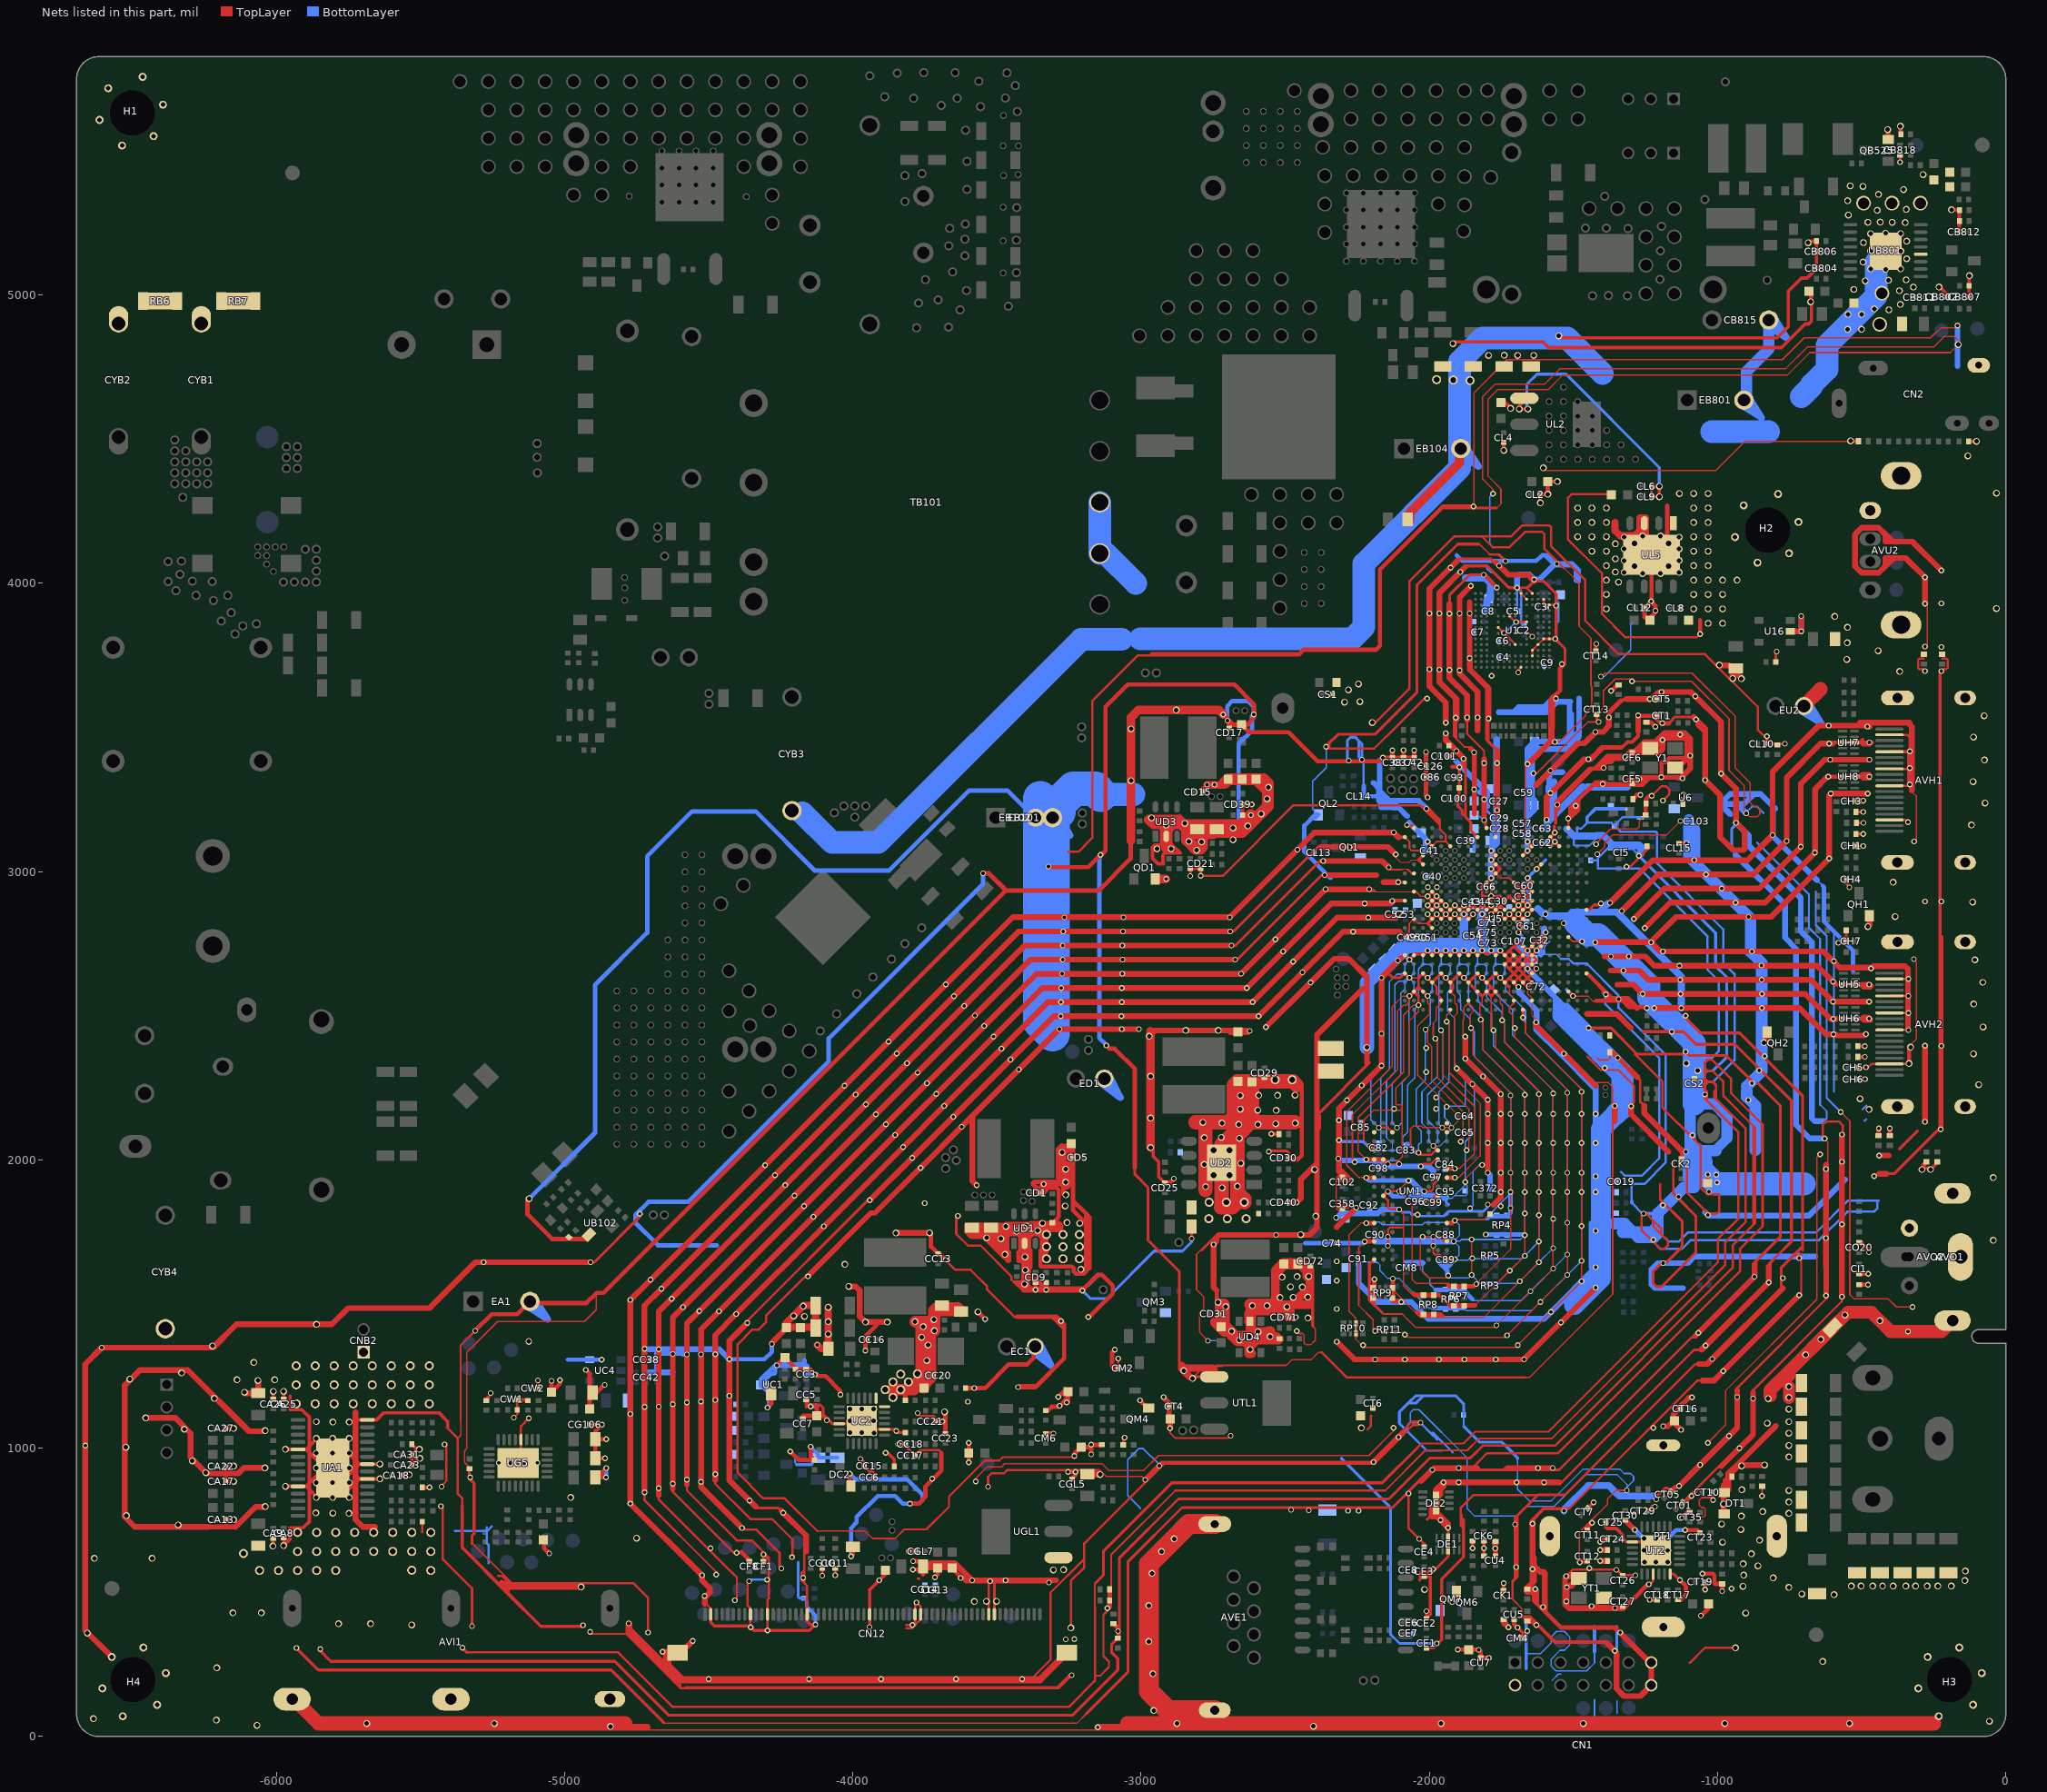
[diagram p0: the nets of this part, all layers, seen from the top]
# Altium PCB MISC84395.PcbDoc (part 18 of 26)
Units mil, origin at the board's own origin, x right, y up, seen from the top; angles counter-clockwise.
Board outline 6692.91 x 5826.77 mil, 2 copper layers (TopLayer, BottomLayer), stack 61.855 mil thick; 951 components, 565 nets, 4374 pads, 1804 vias.
Unrouted connection lines stored in the file: 1.

## Via types
v1: diameter 19.68, hole 11.81, TopLayer to BottomLayer, tented both sides, 1262 vias
v2: diameter 23.62, hole 15.75, TopLayer to BottomLayer, tented both sides, 524 vias
v3: diameter 31.5, hole 19.68, TopLayer to BottomLayer, tented both sides, 11 vias
v4: diameter 24, hole 16, TopLayer to BottomLayer, tented both sides, 6 vias
v5: diameter 19, hole 11.81, TopLayer to BottomLayer, tented both sides, 1 vias

## Nets (pads, with @x,y where several pads share a name; then routed paths per layer and width w, separated by ;. In a path a pad name is that pad's centre, name@x,y a point inside that pad or via, vN(x,y) a via of type N, cw(c..) or ccw(c..) an arc to the next point about the centre after c; other vN are vias at no path point) (continued)
GND: (continued)
  TopLayer w50: AVI1.2@-5931,123 -5853.5,45.5 v2(-5686,45.5) -5276,45.5 ; v2(-5243,45.5) -5276,45.5 ; -4790,45.5 -5276,45.5 ; -3048,45.5 v2(-2876,45.5) v2(-1959,45.5) v2(-1466,45.5) v2(-975,45.5) v2(-543,45.5) -249,45.5 ; -2811.57,2130.91 -2696.31,2130.91 -2678.73,2148.49 -2678.73,2259.08 -2665.51,2272.31 CD26.1@-2664.08,2272.31 ; v2@-2776.83,1896.05 -2776.83,2127.17 -2774,2130 -2679.22,2130 -2660.73,2148.49 -2660.73,2271.77 -2473.34,2271.77 -2460.57,2259 ; -2722.96,1835 -2721,1835 ; pad.VIA5@-2642,1853 -2642,1863.65 -2665.17,1886.83 ; CD28.1@-2615,2258 -2615,2159 -2721,2053 -2721,2033.31 UD2.9@-2721,1990 -2721,1946.69 -2721,1835 ; v2@-2466.98,2130.83 -2618.3,2130.83 -2665.17,2083.95 -2665.17,1886.83 ; EU2.2@-700.62,3574 -700.62,3575.38 -644,3632 ; -2721,1835 -2684,1835 -2665.17,1853.83 -2665.17,1886.83
  TopLayer w70: AVE1.9@-2744.49,91.34 -2906.34,91.34 -2973,158 v2(-2973,330) v2(-2973,454) -2973,598 v2(-2929,642) v2(-2885,686) -2833.99,737.01 AVE1.10@-2744.49,737.01
  BottomLayer w3.94: -2148.9,2077.23 -2128.24,2056.56 -2128.24,2031.45 ; -2120.36,2032.93 -2104.62,2032.93 ; -2085.42,2654.49 -2084.93,2654.98 -2084.93,2678.6 v1(-2069.18,2694.35) -2053.43,2678.6 -2053.43,2647.1 v1(-2069.18,2631.36) ; -2084.93,2591.99 -2084.93,2615.61 v1(-2069.18,2631.36) ; -2053.93,2583.62 -2053.43,2584.11 -2053.43,2615.61 v1(-2069.18,2631.36) ; v1(-2037.69,2536.87) -2037.69,2662.85 -2021.94,2678.6 ; -2021.94,2725.52 -2021.94,2710.1 -2021.94,2678.6 ; v1(-2006.19,2568.36) -1990.44,2584.11 -1990.44,2615.61 v1(-2006.19,2631.36) -1990.44,2647.1 -1990.44,2670.73 -1998.32,2678.6 -2021.94,2678.6 ; -2002.25,2072.3 -2002.25,2088.05 ; v1(-1986.51,2048.68) -1961.9,2048.68 -1939.26,2071.32 -1939.26,2088.37 -1923.51,2104.12 v1(-1923.51,2111.67) ; -1970.76,2072.3 -1970.76,2088.05 ; -1966.82,2562.95 -1966.82,2670.73 -1958.95,2678.6 ; -1958.95,2723.72 -1958.95,2710.1 -1958.95,2678.6 ; -1927.94,2589.52 -1927.45,2590.02 -1927.45,2615.61 v1(-1943.2,2631.36) -1927.45,2647.1 -1927.45,2670.73 -1935.32,2678.6 -1958.95,2678.6 ; -1903.34,2583.13 -1903.83,2583.62 -1903.83,2670.73 -1895.95,2678.6 ; -1895.95,2725.78 -1895.95,2710.1 -1895.95,2678.6 ; -1863.97,2560.98 -1864.46,2561.47 -1864.46,2615.61 v1(-1880.21,2631.36) -1864.46,2647.1 -1864.46,2670.73 -1872.33,2678.6 -1895.95,2678.6 ; -1840.34,2581.65 -1840.84,2582.14 -1840.84,2670.73 -1832.96,2678.6 ; -1832.96,2725.83 -1832.96,2710.1 -1832.96,2678.6 ; -1801.96,2592.48 -1801.47,2592.97 -1801.47,2615.61 v1(-1817.21,2631.36) -1801.47,2647.1 -1801.47,2670.73 -1809.34,2678.6 -1832.96,2678.6 ; -1777.35,2585.1 -1777.84,2585.59 -1777.84,2670.73 -1769.97,2678.6 ; -1769.97,2725.39 -1769.97,2710.1 -1769.97,2678.6 ; v1(-1754.22,2631.36) -1738.47,2647.1 -1738.47,2670.72 -1746.35,2678.6 -1769.97,2678.6
  BottomLayer w4.92: C91.1@-2244.87,1634.98 -2234.71,1645.14 -2180.89,1645.14 -2171.05,1635.3 -2171.05,1615.61 -2143.98,1588.54 -2104.61,1588.54 -2001.27,1485.2 -1987.41,1485.2 ; v1(-2218.79,1780.96) -2214.85,1784.9 -2173.51,1784.9 -2164.16,1775.55 -2023.41,1775.55 -2016.03,1782.93 -1918.59,1782.93 v1(-1911.7,1789.82) ; -2180.86,2008.74 -2167.75,1995.64 -2161.56,1995.64 -2159.99,1997.21 -2103.63,1997.21 ; v1(-2175.48,2111.67) -2203.04,2139.23 -2203.04,2279.98 -2158.75,2324.27 -2158.75,2629.39 -2093.79,2694.35 ; -2148.9,2077.23 -2148.9,2275.06 -2119.38,2304.59 -2119.38,2607.25 -2106.54,2620.08 -2089.25,2620.08 -2077.97,2631.36 v1(-2069.18,2631.36) ; -2120.36,2032.93 -2124.3,2032.93 -2125.78,2031.45 -2128.24,2031.45 -2153.17,2031.45 -2170.4,2048.68 -2175.48,2048.68 -2168.59,2055.57 -2168.59,2284.9 -2139.06,2314.43 -2139.06,2617.08 -2112,2644.15 -2095.76,2644.15 -2085.42,2654.49 ; -2104.62,2032.93 -2103.63,2032.93 -2092.8,2043.76 -2092.8,2079.19 -2075.09,2096.91 -2075.09,2260.29 -2050.48,2284.9 -2050.48,2524.07 v1(-2037.69,2536.87) ; -2084.93,2591.99 -2099.69,2577.22 -2099.69,2294.74 -2129.22,2265.21 -2129.22,2128.4 v1(-2112.49,2111.67) -2094.77,2129.39 -2094.77,2270.14 -2070.17,2294.74 -2070.17,2567.38 v1(-2069.18,2568.36) -2053.93,2583.62 ; v1(-2037.69,2025.06) -2037.69,2052.37 -2027.84,2062.21 -2027.84,2099.86 -2045.56,2117.58 -2045.56,2245.53 -2013.57,2277.52 v1(-2013.57,2452.22) -1996.35,2469.45 -1996.35,2558.52 v1(-2006.19,2568.36) ; -2023.41,1642.68 -2023.41,1613.15 -1998.31,1588.05 -1998.31,1568.37 -1979.12,1549.17 ; -2002.25,2072.3 -2002.25,2064.43 v1(-1986.51,2048.68) -1970.76,2064.43 -1970.76,2072.3 ; -2002.25,2088.05 -2002.25,2103.8 -2025.88,2127.42 -2025.88,2235.69 -1971.74,2289.82 -1971.74,2412.85 v1(-1979.12,2420.23) ; -1970.76,2088.05 -1970.76,2101.83 -2006.19,2137.26 -2006.19,2225.84 -1952.06,2279.98 -1952.06,2442.38 -1966.82,2457.14 -1966.82,2562.95 ; v1(-1955.01,2111.67) -1966.82,2123.48 -1966.82,2235.69 -1932.37,2270.14 -1932.37,2471.91 v1(-1939.75,2479.29) ; C95.1@-1942.21,1867.18 -1942.96,1867.18 -1943.2,1866.95 -1942.21,1866.96 -1921.54,1867.18 -1913.65,1875.07 ; v1(-1934.83,1598.38) -1927.45,1591.01 -1863.47,1591.01 v1(-1853.63,1600.85) -1824.1,1571.32 RP3.5@-1806.38,1571.32 ; -1927.94,2589.52 -1937.29,2580.17 -1937.29,2516.2 -1912.69,2491.59 -1912.69,2334.11 -1843.79,2265.21 -1843.79,2095.43 -1848.8,2090.42 -1875.77,2063.45 -1875.77,1912.96 -1886.74,1901.99 -1913.65,1875.07 ; v1(-1923.51,2111.67) -1926.96,2115.12 -1926.96,2126.93 -1947.14,2147.1 -1947.14,2178.91 -1939.58,2186.47 -1875.97,2186.47 -1875.97,2287.55 v1(-1905.3,2316.89) ; -1903.34,2583.13 -1893,2572.79 -1893,2545.73 -1890.54,2543.27 -1890.54,2521.12 -1858.55,2489.13 -1858.55,2459.6 -1843.79,2444.84 -1843.79,2358.72 -1718.3,2233.23 -1718.3,1883.82 -1757.66,1844.45 -1784.24,1817.88 -1809.34,1792.78 -1801.46,1792.78 -1797.53,1796.71 ; -1880.7,1485.2 -1873.31,1477.82 -1644.48,1477.82 v1(-1472.23,1650.06) -1472.23,2245.53 -1666.62,2439.92 -1666.62,2518.66 ; -1868.47,1912.75 -1868.47,1881.22 -1874.29,1875.4 -1913.32,1875.4 -1913.65,1875.07 ; -1863.97,2560.98 -1861.01,2558.03 -1861.01,2535.88 -1821.64,2496.51 v1(-1821.64,2486.67) -1814.26,2479.29 -1814.26,2380.86 -1669.08,2235.69 v1(-1669.08,1738.64) -1683.84,1723.88 -1888.08,1723.88 -1893.98,1717.97 v1(-1915.64,1717.97) ; v1(-1858.55,1832.15) -1848.71,1841.99 -1848.71,1960.1 -1826.56,1982.24 v1(-1816.72,1982.24) ; -1840.34,2581.65 -1831.49,2572.79 -1831.49,2550.65 -1784.73,2503.89 -1784.73,2457.14 v1(-1777.35,2449.76) -1777.35,2395.63 -1619.87,2238.15 v1(-1619.87,1716.5) v1(-1669.08,1667.28) -1678.92,1657.44 RP5.4@-1763.08,1657.44 ; -1809.34,1792.77 -1908.75,1792.77 v1(-1911.7,1789.82) ; RP5.3@-1806.38,1657.44 -1861.01,1657.44 -1865.93,1652.52 -1909.23,1652.52 v1(-1911.7,1654.98) -1897.92,1668.76 -1897.92,1700.26 v1(-1915.64,1717.97) ; -1801.96,2592.48 -1801.96,2565.41 -1747.82,2511.28 v1(-1747.82,2484.21) -1740.44,2476.84 -1740.44,2410.56 -1570.66,2240.77 v1(-1570.66,1694.35) v1(-1619.87,1645.14) -1693.69,1571.32 RP3.6@-1763.08,1571.32 ; -1777.35,2585.1 -1710.91,2518.66 -1710.91,2432.54 -1521.45,2243.08 v1(-1521.45,2233.23) ; v1(-1754.22,2631.36) -1735.52,2612.67 -1735.52,2587.56 -1666.62,2518.66 ; -1681.38,1512.27 v1(-1521.44,1672.21) v1@-1521.45,2232.08 ; v1@-1666.62,2493.56 -1666.62,2518.66 ; v1(-1915.64,1717.97) -1895.46,1738.15 -1895.46,1773.59 v1(-1911.7,1789.82)
  BottomLayer w5: v1(-2768.12,1372.82) -2740.3,1372.82 ; QL2.E@-2385.5,3197 -2404.75,3216.25 -2404.75,3313.66 -2398.89,3319.52 -2398.69,3319.52 -2358.03,3360.18 v1(-2358.03,3432.68) -2358.03,3398.38 ; v1(-2106.92,1038.59) -2081.76,1063.76 -2074.84,1070.67 -2073.34,1072.17 -2073.34,1080.3 -2073.34,1084.87 -2066.66,1091.55 -2066.66,1123.13 -2056.18,1133.61 -2036.46,1133.61 -1876.41,973.56 -1869.34,966.49 -1869.34,790.67 -1843.18,764.51 -1696.82,764.51 -1663.83,797.5 -1568.36,797.5 -1458.06,907.8 -1348.27,907.8 -1315,874.53 -1315,864.47 ; -1881.27,1083.55 -1881.27,1087.27 ; -1851.28,1517.76 -1845.91,1512.38 -1681.27,1512.38 v1(-1649.4,1544.25) ; -1826.65,3191.74 -1813.43,3178.52 v1(-1810.13,3178.52) ; v1(-1779,4311) -1790.55,4299.45 -1790.55,4137.03 -1780.18,4126.66 -1771,4126.66 ; -1750.83,1020.21 -1694,963.38 -1694,885 -1694,858 -1653.5,817.5 -1576.64,817.5 -1466.35,927.8 -1339.99,927.8 -1324.53,912.34 -1301.82,912.34 -1291.66,902.18 -1291.66,887.82 -1315,864.47 ; -1664,288 -1614,288 -1577.78,324.22 -1577.78,345.41 -1558.74,364.44 -1531.81,364.44 -1512.78,345.41 -1512.78,318.48 -1531.81,299.44 -1546.56,299.44 -1577.88,268.12 -1577.88,244.42 -1561.05,227.59 -1454.46,227.59 -1427,255.05 -1427,294 ; v1@-1643.06,3344.69 v1(-1638.71,3340.34) ; v1(-1628.24,2725.85) -1615.27,2712.88 -1613.82,2712.88 -1607,2712.88 ; -1582.59,2758.33 -1600.99,2739.92 -1600.99,2718.89 -1607,2712.88 ; -1574,195 -1552,217 -1543,217 ; -1544.89,2696.9 -1544.89,2697.99 -1559.27,2712.37 -1573.63,2712.37 -1574.26,2711.74 -1587.7,2711.74 -1588.85,2712.88 -1607,2712.88 ; v1@-1521.45,2232.08 v1(-1521.45,2233.23) ; -1427,63 -1427,128 ; v1@-1406.83,3675 -1395.12,3675 -1301.83,3768.28 -1301.83,3856.17 -1295,3863 ; -1353.02,845.98 -1323.02,845.98 v1(-1315,854) -1315,864.47 ; -1349,79 -1349,124 ; -643.79,2191.41 -621.82,2169.43 -621.82,2142.18 -622,2142 -623.26,2142
  BottomLayer w6: v1(-4217,989) -4200.31,972.31 -4200.31,950.31 -4195,945 -4142.12,945 CC29.2@-4120.05,967.06 ; -3002.5,791.5 -3046.29,835.29 -3046.29,960.23 -3007.71,998.82 -2992.92,998.82 -2936.63,942.52 v1(-2936.63,938.81) ; -1498.65,3093.24 -1495.15,3089.74 -1445.65,3089.74 -1419.2,3116.19 ; v1@-1471.65,2756.3 v1(-1470.58,2757.37) ; -655.59,2970.25 -635.46,2950.12 -635.46,2824.84 -597,2786.39 v1(-597,2689) -597,2236
  BottomLayer w7: -1881.27,1148.73 -1881.27,1126 ; -1881.27,1152.35 -1881.27,1126 ; v1(-1785.72,2915.3) v1@-1785.72,2918.22 ; -1751.54,1019.5 -1826.19,1019.5 -1881.27,1074.58 -1881.27,1076.7 RM14.2@-1881.27,1116 -1881.27,1126 ; -1729.71,3835.34 v1(-1699.21,3865.84) v1@-1699.21,3869.34 ; v2@-1074.73,2308.93 -1016.28,2308.93 ; v1(-900.83,3202) -900.83,3206 -881.49,3225.34 -863.24,3225.34 -840.81,3202.91 ; -862.81,3100.39 -682.96,2920.55 -682.96,2805.17 -644.5,2766.71 -644.5,2191.41 -643.79,2191.41 ; -659.96,2930.07 -659.96,2814.69 -621.5,2776.24 -621.5,2214.65 v1(-573.12,2166.27) ; -497.58,2175.14 -484,2188.72 ; -490,2136.13 -485,2141.13
  BottomLayer w8: -5380,713 -5270.26,713 ; -5270.26,726 -5270.26,713 ; -5263.94,600.68 -5263.94,665.11 -5270.26,671.43 -5270.26,710.74 ; -5252,729 -5268,713 ; v1@-4354,545 v1@-4301.18,545 ; v1@-4158,1598.18 v1(-4155.69,1595.87) ; v1(-2234,3388) -2229,3383 -2229,3309 ; -2216.65,2463.74 -2216.65,2614.74 -2216.65,2642.74 -2102.05,2757.34 ; RL10.2@-2155,3222.73 -2155,3235.39 -2155,3245.38 ; -2154.64,2658.26 -2154.64,2652.88 -2149.87,2648.11 ; v1@-2030,1090 -2063.65,1090 -2073.34,1080.3 -2074.84,1078.8 -2074.84,1070.67 -2074.84,1056.84 -2010.16,992.16 -1957.2,992.16 ; v1@-2028,1085 -1996,1053 ; -1972.84,1029.84 -1996,1053 ; -1919.49,986.23 -1986.26,1053 -1996,1053 ; C5.1@-1687.91,3902.74 -1695.65,3910.47 v1(-1695.65,3984.74) -1682.21,3971.3 -1682.21,3864.18 C2.1@-1671.48,3853.45 ; -1544.17,2696.9 -1516.07,2696.9 -1500.68,2681.51 -1454.62,2681.51 -1343.65,2570.53 v1(-1343.65,2557.74) -1343.65,2527.38 -1179.8,2363.54 -1179.8,1991.26 -1254.42,1916.65 -1291.35,1916.65 -1298.84,1909.16 -1298.84,1851.84 -1298.14,1851.14 -1261,1814 v1(-1257,1814) ; -1498.65,3093.24 -1498.65,3111.74 -1487.65,3122.74 -1487.65,3148.54 -1473.49,3148.54 -1452.45,3169.58 -1368.22,3169.58 RI12.2@-1358.38,3159.74 ; R26.1@-1440.91,3038.74 -1415.65,3038.74 ; v1(-1387.65,2573.74) -1390.65,2570.74 -1390.65,2541.86 -1202.8,2354.01 -1202.8,2005.2 -1263,1945 -1321.38,1945 -1334.38,1958 ; v1@-1272.45,3051.55 -1272.45,3052.54 -1272.45,3056.06 -1298.6,3082.2 -1353.18,3082.2 -1380.18,3082.2 -1414.65,3047.74 -1414.65,3010.46 -1269.96,3010.46 -1035.65,2776.14 -1035.65,2660.76 -996.3,2621.42 -996.3,2376.79 -1019.08,2354.01 -1067,2354.01 ; GND_JP2.JP_2K@-1267.6,3186 -1269.6,3188 -1330.12,3188 RI12.2@-1358.38,3159.74 ; v1@-1223,1715.35 -1198.94,1691.29 -1123.77,1691.29 -1092.9,1722.16 -648.02,1722.16 -549.58,1820.6 -457.32,1820.6 -445.72,1832.2 -445.72,1855.28 ; -1183,1729.79 -1170.5,1717.29 -1134.54,1717.29 ; -1160,1717.29 -1134.54,1717.29 ; -1147.43,1888.92 -1147.43,1897.52 ; -1115.8,3173.95 -1115.8,3044.39 -901.46,2830.04 -901.46,2714.66 -863.3,2676.51 -863.3,2388.52 ; -1062.6,2270.79 -1016.24,2270.79 -941.3,2345.73 -941.3,2644.2 -980.34,2683.23 -980.34,2798.61 -1209.8,3028.08 -1209.8,3134.9 -1213.65,3138.74 -1337.38,3138.74 RI12.2@-1358.38,3159.74 ; -442.01,1859 -547.94,1859 -658.79,1748.16 -1103.67,1748.16 -1134.54,1717.29 ; v1@-341.37,2629.84 v1@-338.37,2629.84 ; v1@-340.37,3171.16 v1(-339.37,3171.16) ; -5270.26,710.74 -5270.26,713 ; -5270.26,710.74 -5268,713 ; -5270.26,713 -5268,713
  BottomLayer w9.35: v1(-2104.62,1828.21) -2103.98,1828.21 -2093.61,1817.84 -2067.27,1817.84 -2059.43,1810 v1(-2040.64,1810) -2035.72,1805.08 -1949.6,1805.08 -1932.37,1822.3 -1811.74,1822.3 -1799.5,1834.55 v1@-1799.5,1843.95 ; C95.1@-1943.2,1866.95 -1942.21,1866.59 -1942.21,1854.29 -1932.37,1844.45
  BottomLayer w10: v1(-5256,1191) v1@-5251,1191 ; -4190,605 -4190,485 -4184.54,479.54 RG30.2@-4169,479.54 ; v1@-3637,1807.27 v1(-3635.89,1806.16) ; v1(-3204,1547) -3176.08,1519.08 -3118.79,1519.08 -2954.37,1683.5 -2856.37,1683.5 -2824.94,1714.93 v1(-2824.94,1726.94) ; -2413,1607.26 -2412,1608.26 ; v1(-2358.03,3432.68) v1@-2352.84,3432.68 ; v1(-2313.77,2068.36) -2311.31,2068.36 -2306.19,2063.25 -2229.42,2063.25 -2214.85,2048.68 -2175.48,2048.68 ; -2305,965 -2134.84,794.84 -2134.84,354.56 -2103.29,323 v1(-1975,323) ; -2284.84,3399.16 -2284.84,3454.22 ; v1(-2279.89,3384.84) -2284.84,3389.79 -2284.84,3454.22 ; v1(-2218.79,1938.44) v1@-2218.3,1937.95 ; C83.1@-2080.99,2057.18 -2073.75,2057.18 -2055.01,2038.44 -2055.01,2029.78 -2050.28,2025.06 v1(-2037.69,2025.06) ; -2074.84,1056.84 -2081.76,1063.76 -2103.84,1085.84 -2103.84,1125.52 -2072.36,1157 ; -2071.88,3171.24 -2070.35,3169.71 ; C95.1@-1942.21,1866.59 -1942.21,1866.96 C95.1@-1942.21,1867.18 ; v1(-1906.07,3418.31) -1881.15,3393.39 -1881.15,3356.97 -1881.15,3349.9 -1806.22,3274.97 -1804.15,3272.9 -1804.15,3214.75 -1780.28,3190.88 -1780.28,3137.5 ; v1(-1896,3362) v1@-1895.45,3362 ; -1881.27,1076.7 -1825.56,1021 -1748.09,1021 -1710.54,983.46 ; RM14.2@-1881.27,1116 -1881.27,1154.47 -1908.64,1181.84 -2020.16,1181.84 ; v1(-1785.72,3072.3) -1785.72,3132.07 -1780.28,3137.5 ; C28.1@-1766.47,3151.31 -1780.28,3137.5 ; v1(-1697,882) v1@-1694,885 ; -1696.5,969.41 -1710.54,983.46 ; -1694.7,2741.7 -1678.84,2725.85 ; -1694,963.38 -1694,966.91 -1710.54,983.46 ; v1(-1691.23,2788.84) -1679.57,2777.19 -1679.57,2749.12 -1666.22,2735.77 ; -1667.66,2691.89 -1660.42,2699.14 -1660.42,2707.42 -1678.84,2725.85 ; v2@-1662,4604 -1662,4690 -1626.87,4725.13 -1526.13,4725.13 -1206.5,4405.5 -1202.37,4401.37 -1202.37,4362 v2(-1202.37,4336) ; v1(-1659.73,2725.85) -1665.85,2725.85 -1678.84,2725.85 ; v1(-1659.73,2977.82) v1(-1628.24,3009.31) -1596.74,3040.81 ; v1(-1628.47,2663.09) v1@-1628.47,2663.91 ; C105.1@-1628.47,2694.58 C105.1@-1628.24,2694.35 ; v1(-1412.65,3518.74) v1@-1408.8,3522.58 ; v1@-1350,290 -1350,382 ; v1(-1273.45,3055.06) -1273.45,3053.54 -1272.45,3052.54 -1007.34,2787.43 -1007.34,2672.05 -968.3,2633.02 -968.3,2356.91 -1016.28,2308.93 ; -938.62,3058.12 -938.62,3065.19 -950.99,3077.56 -950.99,3148.94 -935.99,3163.94 v1(-935.99,3169.07) ; -2284.84,3454.22 -2273.22,3465.84 -2256.78,3465.84 -2245.16,3454.22 ; -2245.16,3454.22 -2234,3443.06 v1(-2234,3388) -2245.16,3399.16 -2245.16,3454.22 ; -2072.36,1157 -2045,1157 -2020.16,1181.84 ; -2072.36,1157 -2047.52,1181.84 -2020.16,1181.84
  BottomLayer w11.81: RP3.5@-1806.38,1571.32 RP3.6@-1763.08,1571.32 ; RP5.3@-1806.38,1657.44 RP5.4@-1763.08,1657.44 ; -1797.53,1796.71 -1789.65,1804.59
  BottomLayer w12: v1(-4936,386) v1@-4935,385 ; -4195,943.25 -4143.86,943.25 -4142.12,945 ; RG30.2@-4169,479.54 -4160,470.54 -4160,451 ; -4156,447 -4160,451 ; v1(-4146,1005) -4120.05,979.05 CC29.2@-4120.05,967.06 CC30.2@-4054,967.06 ; v1(-4130,388) -4130,421 -4160,451 ; v1(-1850,653) v1@-1849,654 ; R50.2@-1845,3074 -1845,3119 ; v1@-1743,527 v1@-1743,532 ; -1664,236 -1664,288 -1664,391 ; -1524.25,2590.68 v1(-1502.25,2568.68) ; -1453.28,3171.58 -1453.28,3188.58 -1424.46,3217.4 GND_JP1.JP_2K@-1325.6,3217.4 ; -1427,294 -1427,381 ; -1298.14,1851.14 -1298.14,1856.95 ; v1(-1257,1814) -1208.32,1814 ; v1@-1034,1948 v1(-1034,1949) ; v1@-489.22,2396.21 v1@-489.12,2396.21 ; v1@-489.12,2357.91 v1@-489.12,2359.21
  BottomLayer w15: -4988.13,1307.13 UC4.5@-4913.13,1307.13 -4871.13,1307.13 v1(-4871,1307) ; v1(-4856,899) -4856,930 v1(-4855,931) ; v1(-4428.5,1308.5) -4306.4,1308.5 -4280.67,1334.23 v1(-4280.67,1361.67) ; UC1.3@-4315,1220 -4315,1227.87 -4284.08,1258.79 -4272.36,1258.79 -4269.15,1262 -4269.15,1278.43 v1@-4261.83,1285.75 ; v1(-4296,1141) -4290.15,1146.85 -4290.15,1191.15 -4313,1214 -4319,1214 -4319,1238.58 v1@-4271.83,1285.75 ; -4167.24,1258 -4167.24,1278.86 ; -4167.24,1305.76 -4167.24,1291 ; RC3.1@-4157.24,1258 -4146.38,1258 ; -4157.14,1285.75 -4167.24,1285.75 ; v1(-4146,1145) -4131,1145 -4127,1149 ; v1@-4126,1258 -4146.38,1258 ; v1(-4090,1097) v1@-4086.47,1100.53 ; v1(-4010.5,911.5) -3990.5,891.5 -3810.9,891.5 -3758.66,839.25 -3758.66,820.75 -3771.75,807.66 v1(-3802,807.66) -3826.5,807.66 -3853.34,834.5 -3913.5,834.5 -3986.66,761.34 -3986.66,742.5 -4006.15,723.01 v1(-4006.15,624.47) ; v1@-3541,1443.21 v1(-3541,1448) ; v1@-3430.3,1212.3 -3427.3,1212.3 v1(-3427,1212) ; v1@-3324,3018 v1(-3321,3018) ; -3185,1566 -3150,1601 ; v1(-3183,1455) v1@-3182,1454 ; v1(-3141,3058) -3145,3054 -3145,2423.4 v1@-3120,2398.4 ; v1(-3120,2397) v1@-3120,2398.4 ; v1@-3119,2397.4 v1@-3120,2398.4 ; v1(-2700,3523.19) -2701.5,3524.69 -2701.5,3573.42 -2683.42,3591.5 -2629.58,3591.5 -2609,3570.92 v1(-2609,3545) -2615.05,3538.95 -2615.05,3490.28 -2661.77,3443.55 -2661.77,3156.23 ; QL2.E@-2396,3186.5 QL2.E@-2385.5,3197 -2396.21,3197 -2434,3159.21 -2434,3069 -2343,2978 ; -2227.27,3299.27 CL14.1@-2227.27,3261 -2188,3261 ; v1@-2130,3420 v1(-2128,3420) ; v1@-2091,3422 v1(-2090.06,3421.06) ; -2084.49,2709.67 v1(-2069.18,2694.35) ; C41.1@-2014.73,3072 -2014.73,3114.09 C33.1@-2014.73,3120.92 ; -1905.65,4096.74 -1885.99,4077.08 -1628.9,4077.08 -1609.24,4096.74 -1598.05,4096.74 ; -1796.02,4052.84 -1784.44,4041.26 ; -1688.7,2576.66 v1@-1688.7,2591.08 ; -1590.86,4096.74 v1@-1563.86,4069.74 ; -1555.65,3867.74 -1555.65,3931.74 ; -1491.65,4007.74 -1491.65,4048.74 -1504.99,4062.08 -1563.39,4062.08 -1566.35,4065.04 -1598.05,4096.74 ; -1481.87,4005.52 -1481.87,4046.52 -1505.09,4069.74 v1@-1563.86,4069.74 ; R33.1@-1370.65,3082.47 -1353.45,3082.47 -1298.87,3082.47 -1298.6,3082.2 ; v2(-1173.05,686.47) -1143.52,716 v1(-1113,716) ; v1@-1044,510 v1(-1043,510) ; -635.46,2950.12 -630.96,2945.62 -630.96,2826.71 -530.33,2726.08 -530.33,2657 ; v1@-4271.83,1285.75 -4266.58,1291 -4167.24,1291 ; v1@-4271.83,1285.75 v1@-4261.83,1285.75 ; v1@-4261.83,1285.75 -4174.13,1285.75 ; -4174.13,1285.75 -4167.24,1278.86 ; -4174.13,1285.75 -4167.24,1285.75 ; -4167.24,1278.86 -4146.38,1258 ; -4167.24,1278.86 -4167.24,1285.75 ; -4167.24,1285.75 -4167.24,1291 ; -1598.05,4096.74 -1597.86,4096.74 -1570.86,4069.74 v1@-1563.86,4069.74
  BottomLayer w15.75: v2(-5123,1865) -4894,2094 -4894,2607 -4713,2788 -4713,3053 -4557,3209 -4337,3209 -4131,3003 -3875,3003 -3597.61,3280.39 -3462.4,3280.39 -3369,3187 EB102.2@-3366.2,3187 ; -4472,1704 -4676,1704 -4754,1782 -4754,1809 -4709,1854 -4571.52,1854 -4083.3,2342.21 -4083.3,2421.7 -3548,2957 v1(-3548,2994) ; -2431,1711 -2354.21,1711 -2353.33,1711.87 -2229.31,1711.87 v1(-2224.69,1716.49) ; v1@-2218.3,1937.95 -2208.45,1928.11 -2062.78,1928.11 ; v1(-2143.99,1891.2) -2126.27,1873.48 -2087.65,1873.48 ; -2065.68,1873.41 -2065.6,1873.48 ; -2046.77,1892.31 -2065.6,1873.48 ; v1(-2018,1859.7) -2031.78,1873.48 -2065.6,1873.48 ; -1987.41,1485.2 -1880.7,1485.2 ; -1979.12,1549.17 -1883.16,1549.17 -1882.7,1549.17 -1851.28,1517.76 ; v1(-1934.83,1598.38) -1937.29,1600.84 -1937.29,1616.1 -1943.2,1622.01 -1943.2,1631.04 -1934.16,1631.04 -1911.7,1653.51 v1(-1911.7,1654.98) ; v1(-1804.42,1741.1) -1671.53,1741.1 v1(-1669.08,1738.64) ; -1789.65,1804.59 -1730.11,1804.59 -1718.29,1816.4 v1(-1718.29,1888.74)
  BottomLayer w18: v1(-1691.23,2599.86) -1691.23,2582.34 -1629.71,2520.82 v1(-1629.71,2476.83) ; C57.1@-1659.73,3172.55 -1661.92,3174.75 -1661.92,3225.4 -1661.38,3225.93 -1658.98,3228.34 ; -1349.38,3086.01 -1266.15,3086.01 RI9.2@-1264.65,3086.01 -1264.65,3063.86 -1266.15,3062.36 v1@-1272.45,3056.06 ; v1(-1287.73,717) -1287,717 v2@-1256.64,686.64
  BottomLayer w19: -2194,3308 -2176.15,3290.15 -2176.15,3246.09 -2167.66,3237.6 ; v1(-2161.21,3394.79) -2171.9,3384.1 -2171.9,3279.39 ; -2077,3192 -2107.73,3222.73 ; -2070.35,3169.71 -2014.73,3114.09 v1@-2006.19,3105.55 ; v1(-2010,3218) -2037.5,3245.5 -2138.01,3245.5 ; -2171.9,3279.39 -2138.01,3245.5 ; -2171.9,3279.39 -2171.9,3269.03 -2167.66,3264.79 ; -2167.66,3237.6 -2167.55,3237.49 -2167.55,3235.39 ; -2167.66,3237.6 -2167.66,3235.39 -2167.55,3235.39 ; -2167.66,3237.6 -2167.66,3264.79 ; -2167.66,3264.79 -2148.37,3245.5 -2138.01,3245.5 ; -2167.55,3235.39 -2167.55,3222.73 RL10.2@-2155,3222.73 -2107.73,3222.73 ; -2167.55,3235.39 -2155,3235.39 -2120.39,3235.39 -2107.73,3222.73
  BottomLayer w19.68: C91.1@-2244.87,1634.98 -2244.87,1571.32 -2180.89,1507.34 -2062.79,1507.34 ; v1(-2166.13,2631.85) -2149.87,2648.11 -2072.14,2725.84 -2037.69,2725.84 v1(-2006.19,2725.84) v1(-1974.69,2725.84) v1(-1943.2,2725.84) ; CM8.1@-2080.01,1640.53 CM8.1@-2077.86,1642.68 ; -2006.19,1450.75 -2062.79,1507.34 ; v1@-1947.13,2725.85 v1(-1943.2,2725.84) ; v1(-1754.22,2725.85) v1(-1943.2,2725.84) ; -1661.38,3225.93 -1661.38,3255.84 -1659.73,3257.5 v1(-1659.73,3373.19) -1659.73,3426.32 C56.1@-1634.71,3451.34 v1@-1566.25,3451.34 ; v1(-1659.73,3072.3) v1(-1659.73,3103.8) C57.1@-1659.73,3172.55 ; v1@-1655.73,2883.33 v1@-1655.73,2977.82 ; -1639.47,2529.4 -1628.18,2518.1 -1628.18,2462.99 -1423.02,2257.84 v1(-1423.02,2159.41) v1(-1423.02,2058.52) v1(-1423.02,1942.88) v1(-1423.02,1888.74) -1423.02,1795.11 ; -1617.21,3424.79 -1523.88,3424.79 -1480.34,3468.33 -1480.34,3480.17 ; -1600.18,1450.75 v1(-1578.04,1472.89) ; -1514.06,3585.33 -1514.06,3474.42 -1537.13,3451.34 ; -1507.99,3546.4 -1507.99,3472.4 ; -1480.34,3600.16 -1480.34,3487.07 ; -1436.69,1614.25 -1436.69,1626.68 -1437.7,1627.7 -1437.7,1780.43 -1423.02,1795.11 ; -1400.65,1585.58 -1400.65,1688.84 ; -1400.65,1772.74 -1404.83,1776.93 -1423.02,1795.11 ; -2062.79,1507.34 -2004.56,1449.12 -1601.82,1449.12 v1(-1578.04,1472.89) ; v1(-1578.04,1472.89) v1(-1423.02,1627.91) -1423.02,1795.11 ; v1@-1566.25,3451.34 v1(-1564.65,3449.74) -1538.74,3449.74 -1537.13,3451.34 ; v1@-1566.25,3451.34 -1537.13,3451.34 ; -1537.13,3451.34 -1529.04,3451.34 ; -1529.04,3451.34 -1517.22,3451.34 ; -1529.04,3451.34 -1507.99,3472.4 ; -1517.22,3451.34 -1516.06,3451.34 ; -1517.22,3451.34 -1507.99,3460.57 -1507.99,3472.4 ; -1516.06,3451.34 -1509.17,3451.34 -1480.34,3480.17 ; -1516.06,3451.34 -1480.34,3487.07 ; -1480.34,3480.17 -1480.34,3487.07
  BottomLayer w19.69: v1@-2321.15,1797.7 -2306.38,1814.43 -2179.42,1814.43 -2165.64,1828.21 v1(-2104.62,1828.21) ; v1(-2316.23,2004.39) -2313.87,2004.39 -2307.37,1997.89 -2183.36,1997.89 -2183.32,1997.86 -2175.48,1990.02 -2168.99,1990.02 -2156.29,1977.32 -2111,1977.32 ; -2187.38,1986.11 -2178.85,1977.58 -2111.26,1977.58 -2111,1977.32 ; CM8.1@-2077.86,1642.68 -2023.41,1642.68 ; -2062.78,1928.11 -2021.94,1887.27 -2011.11,1876.43 -1964.01,1876.43 -1954.52,1866.95 C95.1@-1943.2,1866.95 ; C97.1@-1986.51,1962.69 -2001.13,1977.32 -2111,1977.32 ; -1961.9,1642.68 -1950.26,1631.04 C89.1@-1943.2,1631.04 ; v1(-1797.03,1955.18) -1789.34,1947.48 C372.1@-1789.34,1899.07 ; v1(-1629.71,2476.83) -1629.71,2464.52 -1629.71,2451.87 -1546.4,2368.56 ; v1(-1533.75,2368.56) -1546.4,2368.56 ; -1423.02,2228 -1423.02,2245.19 -1546.4,2368.56